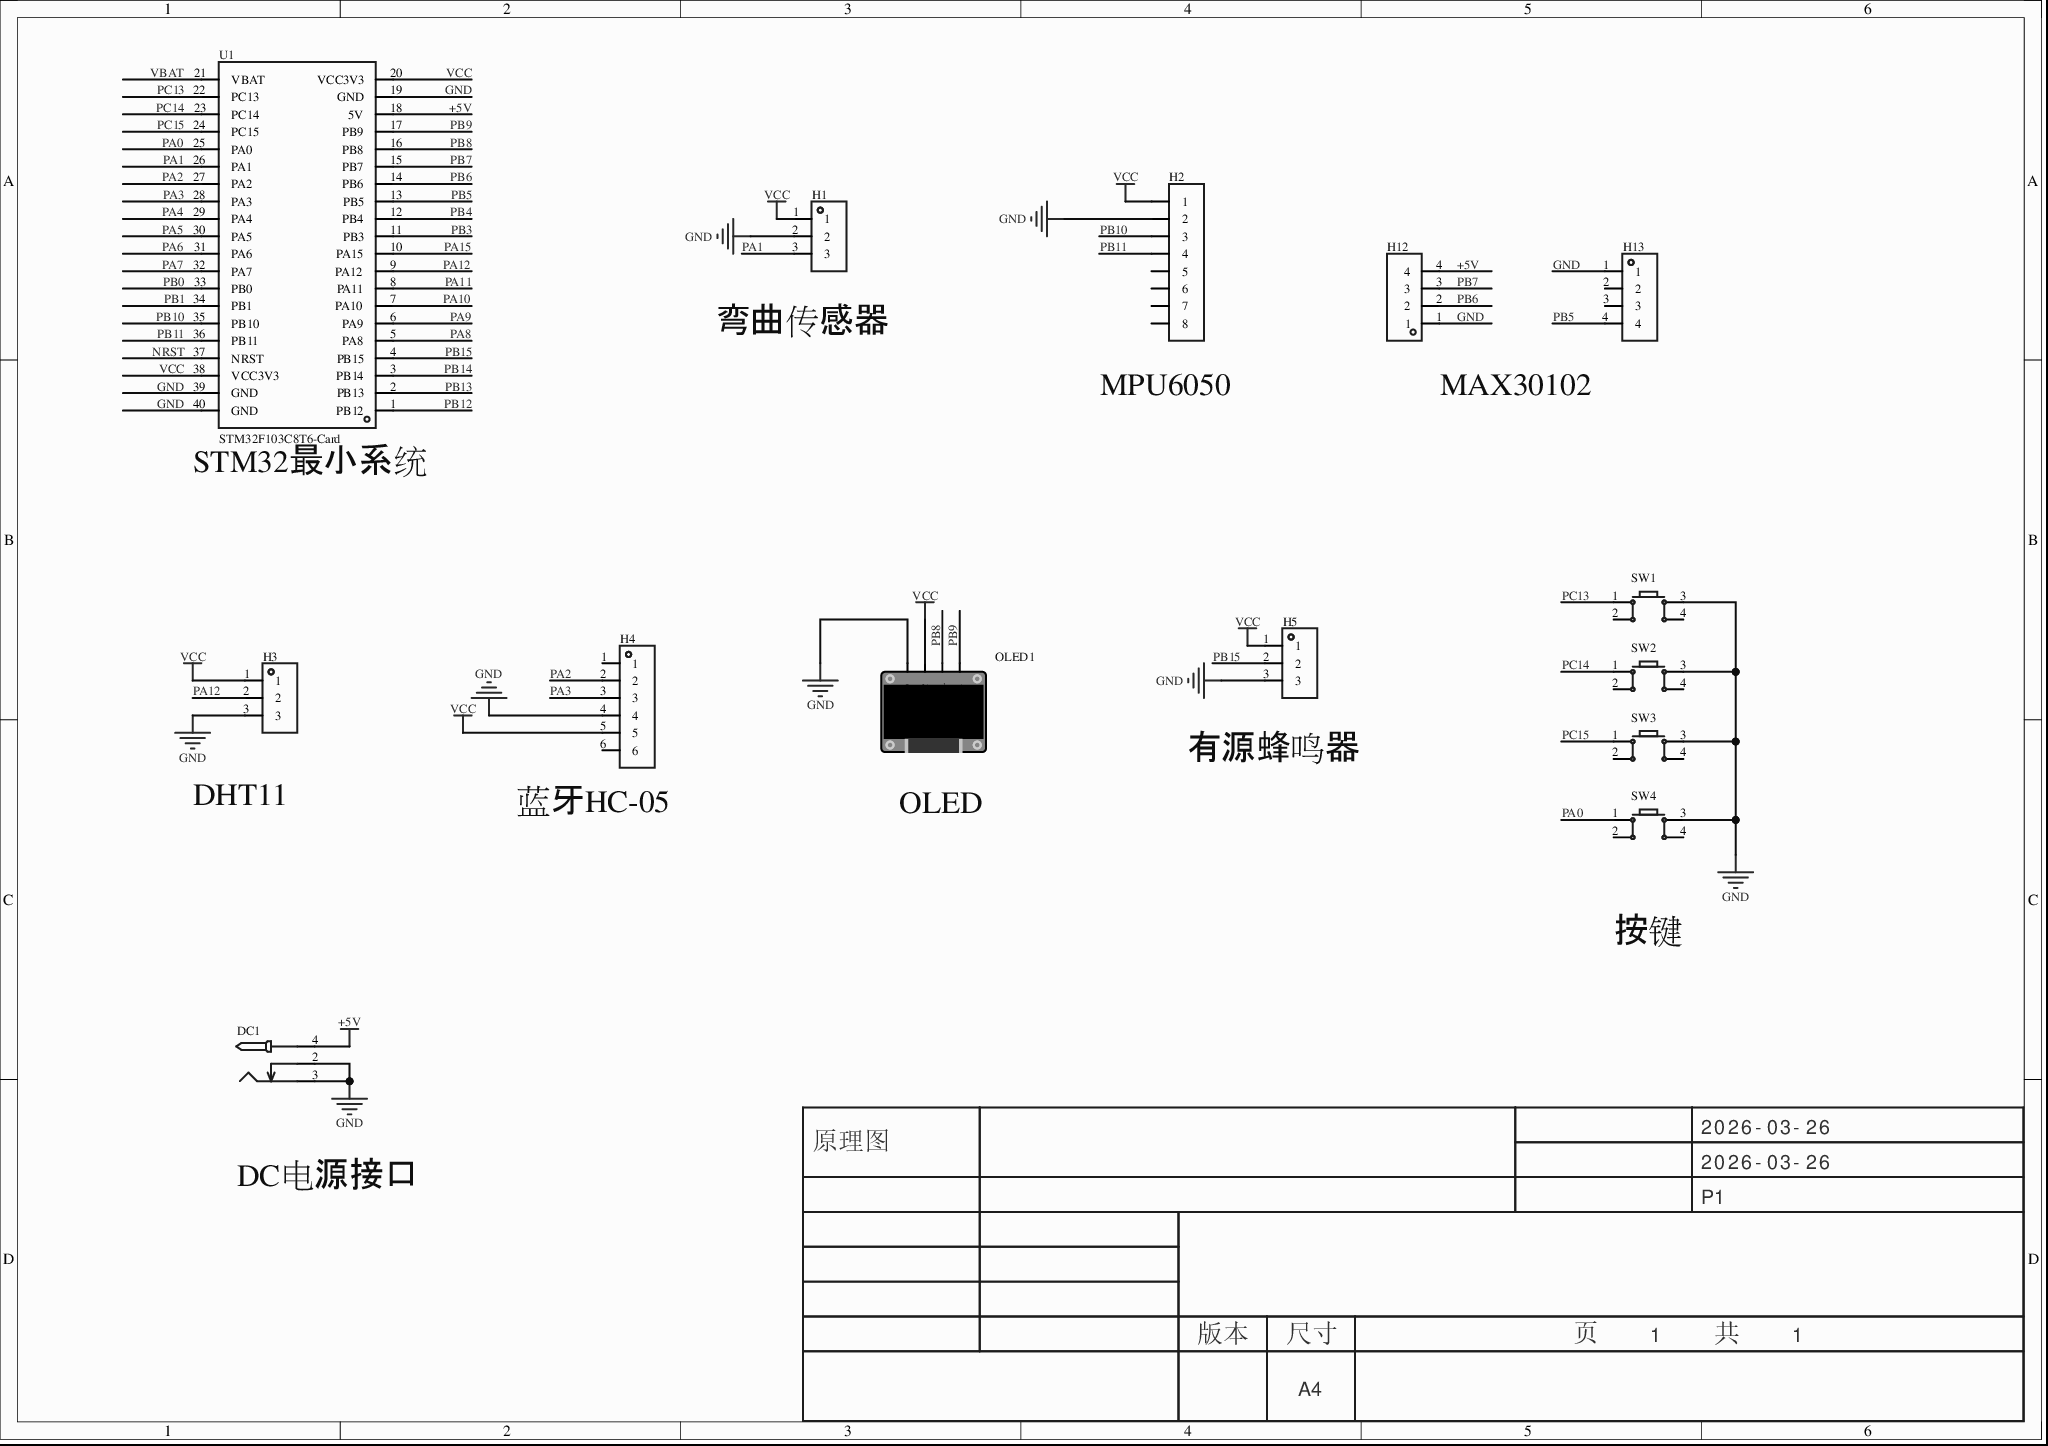
[diagram p0: MISC51890-3.schdoc]
# Altium project MISC51890-2.PrjPcb
1 sheet, 14 parts. Net scope: global (net labels, ports and power ports of the same name join across sheets).
Board file: MISC51890.pcbdoc

## Sheet MISC51890-3.schdoc
size 297 x 209 mm; Version: V1.0; @Project Name: MISC51890; @Page Count: 1; @Update Date: 2026-03-26; @Create Date: 2026-03-26; @Schematic Name: MISC51890; @Page No: 1; @Create Time: 18:58:15; @Update Time: 22:44:58; @Board Name: MISC51890

### Parts
DC1  (no value)  [DC-2.0]
H1  (no value)  [HDR-TH_3P-P2.54-V-F]
H2  (no value)  [HDR-TH_8P-P2.54-V-F-1]
H3  (no value)  [HDR-TH_3P-P2.54-V-F]
H4  (no value)  [HDR-TH_6P-P2.54-V-F]
H5  (no value)  [HDR-TH_3P-P2.54-V-F]
H12  (no value)  [HDR-TH_4P-P2.54-V-F]
H13  (no value)  [HDR-TH_4P-P2.54-V-F]
OLED1  (no value)  [0.96OLED_4P]
SW1  (no value)  [SW-TH_4P-L6.0-W6.0-P4.50-LS6.5]
SW2  (no value)  [SW-TH_4P-L6.0-W6.0-P4.50-LS6.5]
SW3  (no value)  [SW-TH_4P-L6.0-W6.0-P4.50-LS6.5]
SW4  (no value)  [SW-TH_4P-L6.0-W6.0-P4.50-LS6.5]
U1  STM32F103C8T6-Card  [CONN-TH_L53.3-W22.9_STM32F103C8T6-CARD]

### Nets
+5V: DC1.4 H12.4 U1.18(5V)
GND: DC1.2 DC1.3 H1.2 H2.2 H3.3 H4.4 H5.3 H12.1 H13.1 OLED1.1(GND) SW1.3 SW2.3 SW3.3 SW4.3 U1.19(GND) U1.39(GND) U1.40(GND)
VCC: H1.1 H2.1 H3.1 H4.5 H5.1 OLED1.2(VCC) U1.20(VCC3V3) U1.38(VCC3V3)
NRST: U1.37(NRST)
PA0: SW4.1 U1.25(PA0)
PA1: H1.3 U1.26(PA1)
PA2: H4.2 U1.27(PA2)
PA3: H4.3 U1.28(PA3)
PA4: U1.29(PA4)
PA5: U1.30(PA5)
PA6: U1.31(PA6)
PA7: U1.32(PA7)
PA8: U1.5(PA8)
PA9: U1.6(PA9)
PA10: U1.7(PA10)
PA11: U1.8(PA11)
PA12: H3.2 U1.9(PA12)
PA15: U1.10(PA15)
PB0: U1.33(PB0)
PB1: U1.34(PB1)
PB3: U1.11(PB3)
PB4: U1.12(PB4)
PB5: H13.4 U1.13(PB5)
PB6: H12.2 U1.14(PB6)
PB7: H12.3 U1.15(PB7)
PB8: OLED1.3(SCL) U1.16(PB8)
PB9: OLED1.4(SDA) U1.17(PB9)
PB10: H2.3 U1.35(PB10)
PB11: H2.4 U1.36(PB11)
PB12: U1.1(PB12)
PB13: U1.2(PB13)
PB14: U1.3(PB14)
PB15: H5.2 U1.4(PB15)
PC13: SW1.1 U1.22(PC13)
PC14: SW2.1 U1.23(PC14)
PC15: SW3.1 U1.24(PC15)
VBAT: U1.21(VBAT)

Not connected (* = marked no-connect by the designer): H2 5 6 7 8; H4 1 6; H13 2* 3*; SW1 2 4; SW2 2 4; SW3 2 4; SW4 2 4

### Notes on the sheet
- (near H1) 弯曲传感器
- (near H2) MPU6050
- MAX30102
- (near U1) STM32最小系统
- (near H5) 有源蜂鸣器
- (near H3) DHT11
- (near H4) 蓝牙HC-05
- OLED
- 按键
- DC电源接口
- 2026-03-26
- 原理图
- P1
- 版本
- 尺寸
- A4
- 页    1    共    1

### Library data of the parts
DC1 = DC-005_2.0: Symbol: DC电源接口; ConvertToPcb: yes; ModelId: f5f20b8a2308479b936ba3c2698865bb0819f05c4eef4c71ace90d822a990e87; ModelName: DC-IN-TH_DC-5520-1; ModelTransform: 372.05,551.18,582.68,90,0,0,137.8,0,-149.61; Device: DC-005_2.0; AddInBom: yes; Supplier Footprint: 插件; FootprintName: DC-2.0
H1 H3 H5 = HDR-F_2.54_1x3P: Symbol: PM254V-11-03-H85; 3D Model: f3b3cc5aae9641bf9e56fc160cef875b; 3D Model Transform: 299.9994,100,0,0,0,0,0,0,-118.11; ConvertToPcb: yes; ModelName: HDR2.54-F-LI-1X3P; Device: HDR-F_2.54_1x3P; Supplier Part: C541850; Supplier Footprint: 插件; AddInBom: yes; FootprintName: HDR-TH_3P-P2.54-V-F
H2 = HDR-F_2.54_1x8P: Symbol: Header-Female-2.54_1x8; AddInBom: yes; ModelId: 0f7e4d9227ef4fa08d5469c22cc70cdb; ModelName: HDR-F-2.54_1x8; ModelTransform: 799.99844,100,0,0,0,0,0,0,-118.11; Device: HDR-F_2.54_1x8P; ConvertToPcb: yes; FootprintName: HDR-TH_8P-P2.54-V-F-1; SupplierPart: C27438; Supplier Footprint: 插件
H4 = HDR-F_2.54_1x6P: Symbol: Header-Female-2.54_1x6; ConvertToPcb: yes; ModelId: 0f5bcf94dcda47d085f24cdca1696fe9; ModelTransform: 619.684,94.488,0,0,0,0,0,0,-125.984; Device: HDR-F_2.54_1x6P; AddInBom: yes; SupplierPart: C40877; Supplier Footprint: 插件; FootprintName: HDR-TH_6P-P2.54-V-F; ModelName: HDR-TH_6P-P2.54-V-F
H12 H13 = HDR-F_2.54_1x4P: Symbol: 2.54-1*4P母; 3D Model: 57daaad411c24bd7bd5d06edf5c4d16b; 3D Model Transform: 415.7472,98.425,0,0,0,0,0,0,-118.11; ConvertToPcb: yes; ModelName: HDR-TH_4P-P2.54-F-LI-1X4P; Device: HDR-F_2.54_1x4P; Supplier Part: C2718488; Supplier Footprint: 插件; AddInBom: yes; FootprintName: HDR-TH_4P-P2.54-V-F
OLED1 = 0.96OLED模块_4P: ConvertToPcb: yes; ModelId: 79c000fdb68d45a296c2e9bedf4f9055; ModelTransform: 1393.69792,1318.895,0,0,0,0,0,-560.079,-137.795; Symbol: 0.96OLED模块_4P; Device: 0.96OLED模块_4P; AddInBom: yes; FootprintName: 0.96OLED_4P; Supplier Footprint: 插件; ModelName: 0.96OLED_4P
SW1-SW4 = Key_TH_6x6x6: 触点电流:50mA;额定电压(DC):12V;绝缘电阻:100MΩ;电路结构:单刀单掷;安装方式:直插;按钮形状:圆形按钮;按钮/盖帽颜色:黑色;作用力:260gf@±30gf;工作温度:-25℃~+70℃;引脚样式:PC引脚;开关长度:6mm;开关宽度:6mm;开关高度:6mm;带支架:否;; Symbol: 轻触按键; AddInBom: yes; ModelId: 20eee248bc684ccd8cbdbb1d0d91ec6f0819f05c4eef4c71ace90d822a990e87; ModelName: SW-TH_4P-L6.0-W6.0-H5.0-LS6.5-P4.50; ModelTransform: 236.22,323.03,0,90,0,0,0,0,-137.795; Device: Key_TH_6x6x6; ConvertToPcb: yes; FootprintName: SW-TH_4P-L6.0-W6.0-P4.50-LS6.5; Supplier Footprint: 插件
U1 = STM32F103C8T6-Card: AddInBom: yes; Symbol: STM32F103C8T6-CARD; Device: STM32F103C8T6-Card; LCSC Part Name: STM32F103C8T6-Card; SupplierPart: C9900077949; ManufacturerPart: STM32F103C8T6-Card; Supplier Footprint: 插件; Supplier: LCSC; ConvertToPcb: yes; FootprintName: CONN-TH_L53.3-W22.9_STM32F103C8T6-CARD